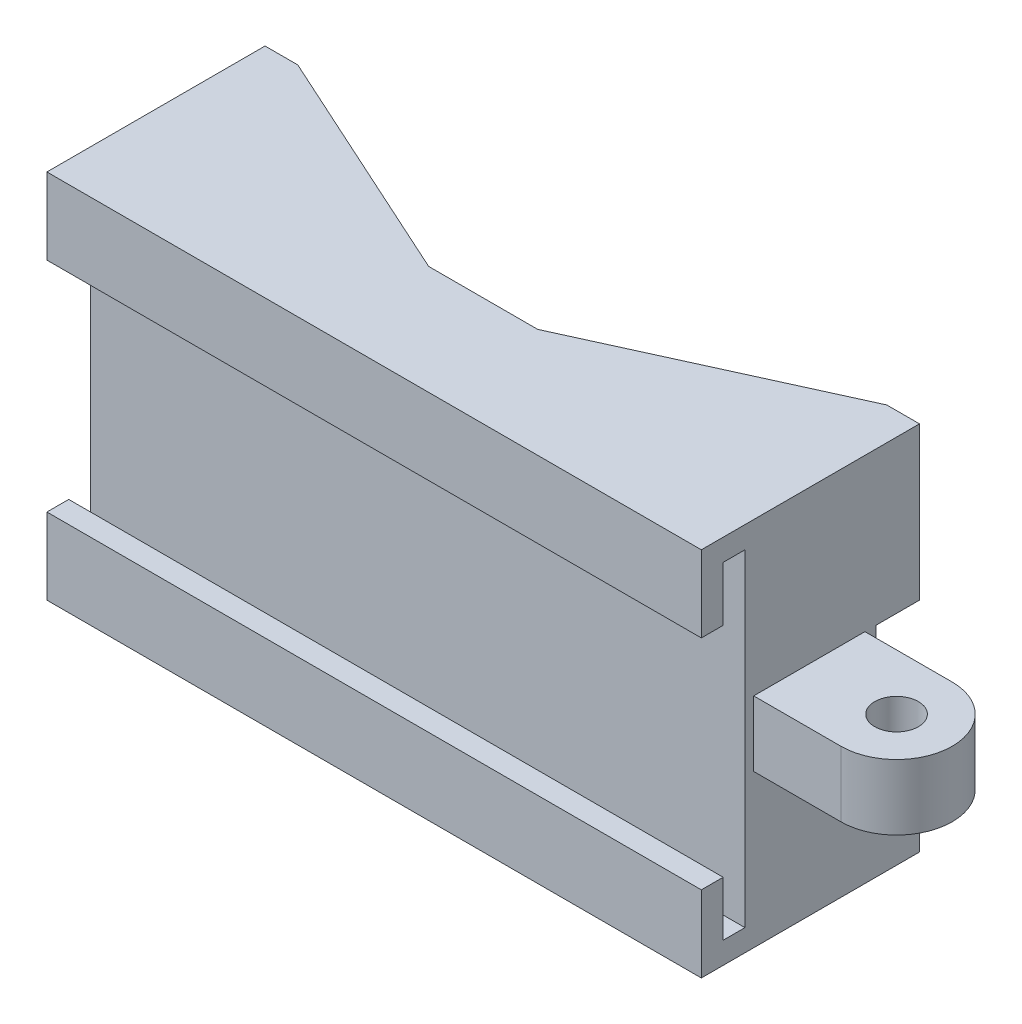
SolidWorks part; units mm, degrees
ref_plane "Front Plane" through (0, 0, 0) normal (0, 0, 1) x (1, 0, 0)
ref_plane "Top Plane" through (0, 0, 0) normal (0, 1, 0) x (1, 0, 0)
ref_plane "Right Plane" through (0, 0, 0) normal (1, 0, 0) x (0, 0, -1)
other "Configuration Table"
sketch "Sketch1" plane through (0, 0, 0) normal (0, 0, 1) x (1, 0, 0)
  line L1 (-150, 85) -> (150, 85)
  line L2 (-150, 85) -> (-150, -85)
  line L3 (-150, -85) -> (150, -85)
  line L4 (150, 85) -> (150, -85)
  line L5 (-150, 85) -> (150, -85) construction
  line L6 (-150, -85) -> (150, 85) construction
  point P0 (0, 0)
  dimension "D1" = 300
  dimension "D2" = 170
extrude "Boss-Extrude1" add sketch "Sketch1" along normal blind 10
sketch "Sketch2" plane through (0, 0, 10) normal (0, 0, 1) x (1, 0, 0)
  line L0 (150, -85) -> (150, 85) construction
  line L1 (-150, 85) -> (150, 85)
  line L2 (-150, 85) -> (-150, 75)
  line L3 (-150, 75) -> (150, 75)
  line L4 (150, 85) -> (150, 75)
  line L6 (-150, -85) -> (150, -85)
  line L7 (-150, -85) -> (-150, -75)
  line L8 (-150, -75) -> (150, -75)
  line L9 (150, -85) -> (150, -75)
  dimension "D1" = 10
  dimension "D2" = 10
extrude "Boss-Extrude2" add sketch "Sketch2" along normal blind 20
sketch "Sketch4" plane through (0, 75, 0) normal (0, -1, 0) x (1, 0, 0)
  line L0 (150, 30) -> (150, 0) construction
  line L1 (-150, 30) -> (150, 30)
  line L2 (-150, 30) -> (-150, 20)
  line L3 (-150, 20) -> (150, 20)
  line L4 (150, 30) -> (150, 20)
  dimension "D1" = 10
extrude "Boss-Extrude3" add sketch "Sketch4" along normal blind 25
mirror "Mirror1" about plane through (0, 0, 0) normal (0, 1, 0) of "Boss-Extrude3"
sketch "Sketch5" plane through (0, 0, 0) normal (0, 1, 0) x (1, 0, 0)
  line L0 (-150, 0) -> (-150, 70)
  line L1 (-150, 70) -> (-135, 70)
  line L2 (-135, 70) -> (-25, 20)
  line L3 (-25, 20) -> (0, 20)
  line L4 (0, 20) -> (0, 0)
  line L5 (-150, 0) -> (0, 0)
  dimension "D1" = 70
  dimension "D2" = 15
  dimension "D3" = 20
  dimension "D4" = 25
extrude "Boss-Extrude4" add sketch "Sketch5" along normal mid plane 170
sketch "Sketch6" plane through (0, 0, 0) normal (0, 1, 0) x (1, 0, 0)
  line L0 (-150, 70) -> (-135, 70)
  line L1 (-135, 70) -> (-25, 20)
  line L2 (-25, 20) -> (0, 20)
  line L3 (0, 20) -> (0, 0)
  line L4 (0, 0) -> (0, 20) construction
  line L5 (0, 0) -> (-25, 0)
  line L6 (-25, 0) -> (-135, 50)
  line L7 (-135, 50) -> (-150, 50)
  line L8 (-150, -30) -> (-150, 70) construction
  line L9 (-150, 50) -> (-150, 70)
  dimension "D1" = 20
extrude "Cut-Extrude1" cut sketch "Sketch6" against normal mid plane 30
mirror "Mirror2" about plane through (0, 0, 0) normal (1, 0, 0) of "Boss-Extrude4", "Cut-Extrude1"
sketch "Sketch8" plane through (0, 0, 0) normal (0, 1, 0) x (1, 0, 0)
  line L0 (150, -30) -> (150, 70) construction
  line L1 (150, -6) -> (190, -6)
  line L2 (150, -6) -> (150, 45)
  line L3 (150, 45) -> (190, 45)
  line L5 (150, -30) -> (-150, -30) construction
  line L6 (135, 70) -> (150, 70) construction
  arc A0 (190, -6) -> (190, 45) centre (190, 19.5) ccw
  circle A1 centre (190, 19.5) radius 10
  dimension "D4" = 20
  dimension "D1" = 24
  dimension "D2" = 25
  dimension "D3" = 40
extrude "Boss-Extrude5" add sketch "Sketch8" along normal mid plane 30
